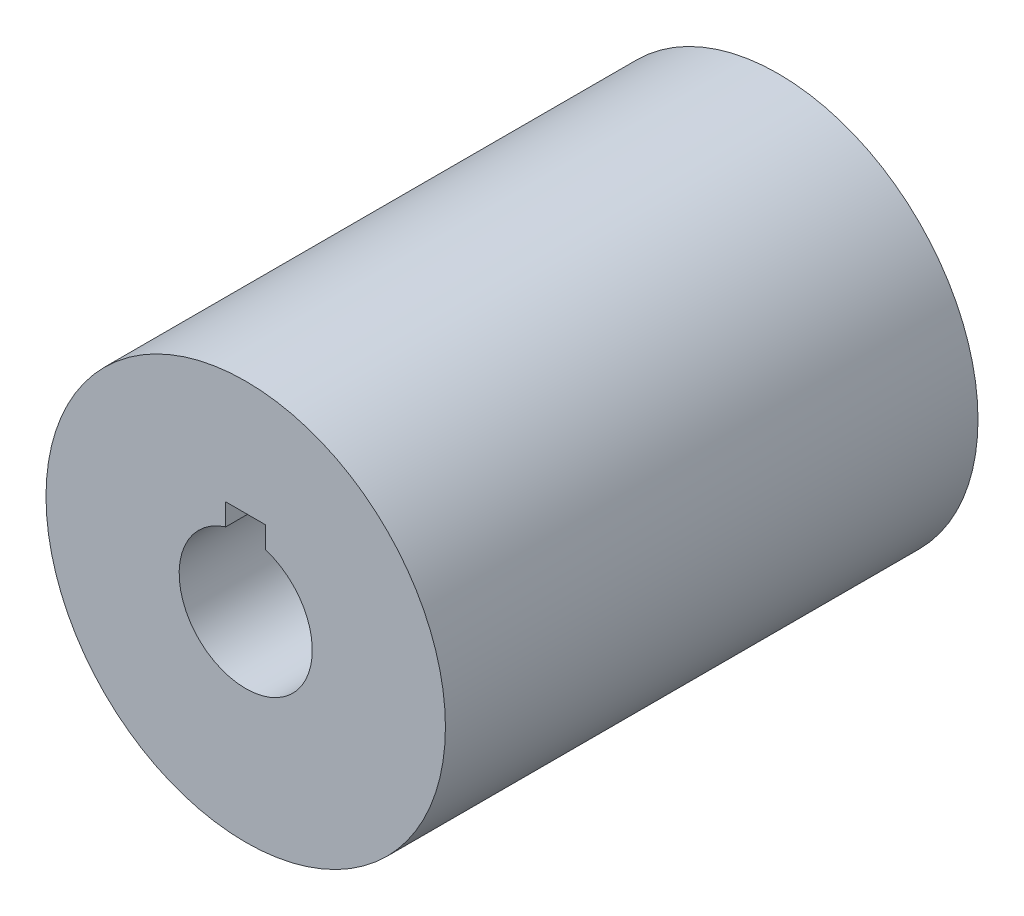
SolidWorks part; units mm, degrees
material "45"
ref_plane "Front" through (0, 0, 0) normal (0, 0, 1) x (1, 0, 0)
ref_plane "Top" through (0, 0, 0) normal (0, 1, 0) x (1, 0, 0)
ref_plane "Right" through (0, 0, 0) normal (1, 0, 0) x (0, 0, -1)
sketch "Sketch1" plane through (0, 0, 0) normal (0, 0, 1) x (1, 0, 0)
  circle A0 centre (0, 0) radius 30
  dimension "D1" = 60
extrude "Boss-Extrude1" add sketch "Sketch1" along normal mid plane 80
sketch "Sketch2" plane through (0, 0, 40) normal (0, 0, 1) x (1, 0, 0)
  circle A0 centre (0, 0) radius 10
  dimension "D1" = 20
extrude "Cut-Extrude1" cut sketch "Sketch2" against normal through all
sketch "Sketch3" plane through (0, 0, -40) normal (0, 0, -1) x (-1, 0, 0)
  circle A0 centre (0, 0) radius 15
  dimension "D2" = 30
extrude "Cut-Extrude2" cut sketch "Sketch3" against normal blind 40
sketch "Sketch4" plane through (0, 0, 40) normal (0, 0, 1) x (1, 0, 0)
  line L0 (0, 0) -> (0, 19.6698) construction
  line L2 (3, 6.8698) -> (-3, 6.8698)
  line L3 (3, 6.8698) -> (3, 12.8)
  line L4 (3, 12.8) -> (-3, 12.8)
  line L5 (-3, 6.8698) -> (-3, 12.8)
  line L6 (0, 12.8) -> (0, 6.8698) construction
  line L7 (3, 9.8349) -> (-3, 9.8349) construction
  circle A0 centre (0, 0) radius 10 construction
  point P3 (0, 9.8349)
  dimension "D1" = 2.8
  dimension "D2" = 6
extrude "Cut-Extrude3" cut sketch "Sketch4" against normal blind 40
sketch "Sketch5" plane through (0, 0, -40) normal (0, 0, -1) x (-1, 0, 0)
  line L0 (0, 0) -> (22.8337, 0) construction
  line L2 (18.3, -4) -> (11.7, -4)
  line L3 (18.3, -4) -> (18.3, 4)
  line L4 (18.3, 4) -> (11.7, 4)
  line L5 (11.7, -4) -> (11.7, 4)
  line L6 (15, 4) -> (15, -4) construction
  line L7 (18.3, 0) -> (11.7, 0) construction
  circle A0 centre (0, 0) radius 15 construction
  point P3 (15, 0)
  dimension "D1" = 3.3
  dimension "D2" = 8
extrude "Cut-Extrude4" cut sketch "Sketch5" against normal blind 40
equation "\"零件重量\"= IIF ( \"SW-质量\" > 100 , int ( \"SW-质量\" ) , \"SW-质量\" )"
